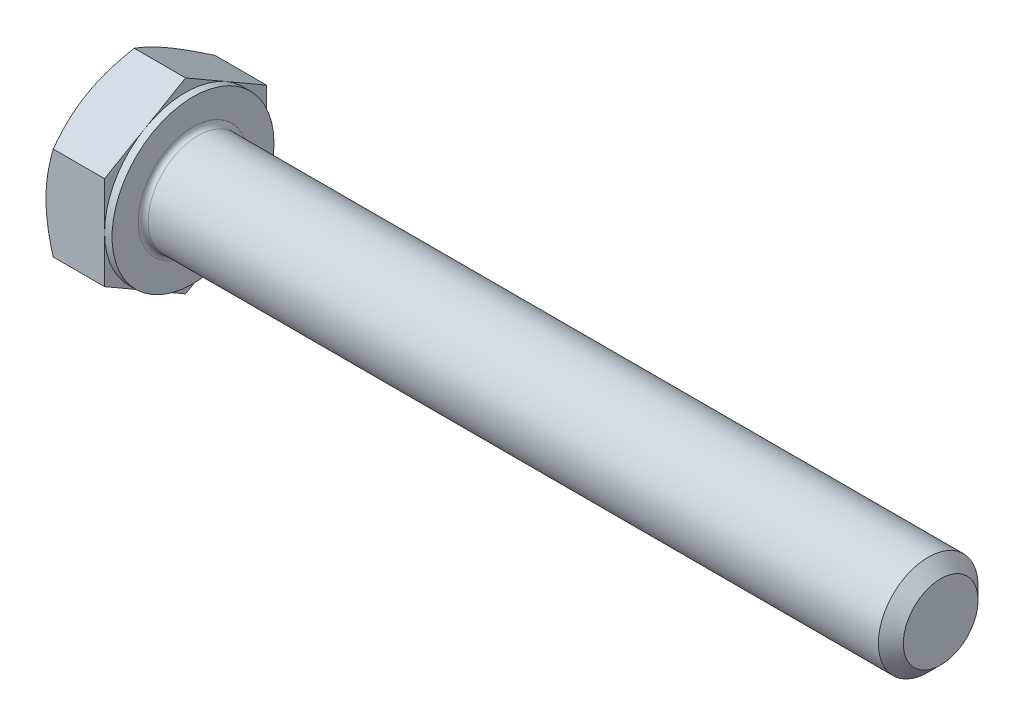
SolidWorks part; units mm, degrees
extrude "Base-Extrude" add sketch "Sketch1" along normal blind 5.3
sketch "Sketch1" plane through (0, 0, 0) normal (1, 0, 0) x (0, 0, -1)
  line L0 (6.5, 3.7528) -> (6.5, -3.7528)
  line L1 (-6.5, 3.7528) -> (-6.5, -3.7528)
  line L2 (6.5, -3.7528) -> (0, -7.5056)
  line L3 (0, -7.5056) -> (-6.5, -3.7528)
  line L4 (6.5, 3.7528) -> (0, 7.5056)
  line L5 (0, 7.5056) -> (-6.5, 3.7528)
revolve "Cut-Revolve1" cut sketch "Sketch3" angle 360 about L6
sketch "Sketch3" plane through (0, 0, 0) normal (0, 0, 1) x (1, 0, 0)
  line L0 (0, 6.5) -> (3.4673, 12.5056)
  line L1 (0, 7.5056) -> (0, 3.7528) construction
  line L2 (3.4673, 12.5056) -> (3.4673, 17.5056)
  line L3 (3.4673, 17.5056) -> (-10, 17.5056)
  line L4 (-10, 17.5056) -> (-10, 6.5)
  line L5 (-10, 6.5) -> (0, 6.5)
  line L6 (0, 0) -> (99.06, 0) construction
  line L7 (5.3, 7.5056) -> (0, 7.5056) construction
ref_plane "Front" through (0, 0, 0) normal (0, 0, 1) x (1, 0, 0)
ref_plane "Top" through (0, 0, 0) normal (0, 1, 0) x (1, 0, 0)
ref_plane "Right" through (0, 0, 0) normal (1, 0, 0) x (0, 0, -1)
sketch "Sketch2" plane through (0, 0, 0) normal (0, 0, 1) x (1, 0, 0)
  line L0 (0, 3.7528) -> (0, -3.7528) construction
  line L1 (0, 0) -> (65.3, 0)
  line L2 (0, 0) -> (0, 4)
  line L3 (0, 4) -> (7.7917, 4)
  line L4 (65.3, 0) -> (65.3, 2.9175)
  line L5 (5.3, 7.5056) -> (5.3, 3.7528) construction
  line L7 (0, 0) -> (96.52, 0) construction
  line L8 (65.3, -2.9175) -> (7.7917, -4) construction
  line L9 (0, -4) -> (7.7917, -4) construction
  line L10 (6.55, 15.24) -> (6.55, -1.27) construction
  line L11 (43.3, 15.24) -> (43.3, -1.27) construction
  line L12 (5.3, 3.7528) -> (5.3, -3.7528) construction
  line L13 (7.7917, 4) -> (65.3, 4)
  line L14 (65.3, 4) -> (65.3, 2.9175)
revolve "Boss-Revolve1" add sketch "Sketch2" angle 360 about L7
cosmetic thread "Helix1" parameters "Thread_length"=22, "Thread_minor"=5.835
sketch "Sketch5" plane through (0, 0, 0) normal (0, 0, 1) x (1, 0, 0)
  line L0 (5.3, 6.5) -> (1.8327, 12.5056)
  line L1 (5.3, 7.5056) -> (5.3, 3.7528) construction
  line L2 (1.8327, 12.5056) -> (1.8327, 17.5056)
  line L3 (1.8327, 17.5056) -> (11.8327, 17.5056)
  line L4 (11.8327, 17.5056) -> (11.8327, 6.5)
  line L5 (11.8327, 6.5) -> (5.3, 6.5)
  line L7 (5.3, 7.5056) -> (0.5806, 7.5056) construction
  line L8 (0, 0) -> (99.06, 0) construction
  line L9 (0, 0) -> (99.06, 0) construction
revolve "Cut-Revolve2" cut sketch "Sketch5" angle 360 about L8
sketch "Sketch4" plane through (0, 0, 0) normal (0, 0, 1) x (1, 0, 0)
  line L1 (5.3, 7.5056) -> (5.3, 3.7528) construction
  line L2 (5.3, 6.5) -> (4.7, 6.5)
  line L3 (5.3, 6.5) -> (5.3, 17.5056)
  line L4 (5.3, 17.5056) -> (4.7, 17.5056)
  line L5 (0, 0) -> (95.25, 0) construction
  line L6 (0, 0) -> (96.52, 0) construction
  line L7 (4.7, 6.5) -> (4.7, 17.5056)
  line L8 (4.7194, 7.5056) -> (0.5806, 7.5056) construction
revolve "Cut-Revolve3" cut sketch "Sketch4" angle 360 about L5
chamfer "Chamfer" distance 1 angle 45 1 edges at (65.3, 0, 4)
fillet "Fillet" radius 0.4 1 edges at (5.3, 0, -4)
sketch "Sketch6" plane through (0, 0, 0) normal (0, 0, 1) x (1, 0, 0)
  line L0 (43.3, -2.9175) -> (42.675, -4)
  line L1 (43.3, -2.9175) -> (43.925, -4)
  line L2 (43.925, -4) -> (43.925, -5)
  line L3 (-3.175, 0) -> (5.1513, 0) construction
  line L5 (43.925, -5) -> (42.675, -5)
  line L6 (42.675, -5) -> (42.675, -4)
revolve "Cut-Revolve4" [suppressed] cut sketch "Sketch6" angle 360 about L3
pattern_linear "LPattern1" [suppressed]
equation "\"D3@Sketch1\" = \"s@Sketch1\" / 2"
equation "\"D4@Sketch1\" = \"D3@Sketch1\""
equation "\"D5@Sketch1\" = \"D4@Sketch1\""
equation "\"Thread_minor@Helix1\" = \"Minor_dia@Sketch2\""
equation "\"D1@Sketch3\" = \"s@Sketch1\" / 2"
equation "\"D1@Sketch5\" = \"s@Sketch1\" / 2"
equation "\"Head_ch_ang@Sketch5\" = \"Head_ch_ang@Sketch3\""
equation "\"D1@Sketch4\" = \"s@Sketch1\""
equation "\"Thread_length@Helix1\" = ((sgn( (\"l@Sketch2\" - \"p@Sketch2\" ) - \"h@Sketch2\" )-1)*( (\"l@Sketch2\" - \"p@Sketch2\" ) - \"h@Sketch2\" ))/-2+ \"h@Sketch2\""
equation "\"Thread_minor@Sketch6\" = \"Minor_dia@Sketch2\""
equation "\"Diameter@Sketch6\" = \"m@Sketch2\""
equation "\"Overcut@Sketch6\" = \"m@Sketch2\" * 1.25"
equation "\"Start@Sketch6\" = \"k@Base-Extrude\" + \"l@Sketch2\" - \"Thread_length@Helix1\"  '---Non-countersunk---"
equation "\"Num_threads@LPattern1\" = int( \"Thread_length@Helix1\" / \"p@Sketch2\" + 0.999 )  + 1"
equation "\"Advance@LPattern1\" = \"Thread_length@Helix1\" /  (\"Num_threads@LPattern1\" - 1) 'relax it"
equation "\"Num_threads@LPattern1\" = \"Num_threads@LPattern1\" - sgn( \"Num_threads@LPattern1\" - 1) '---chamfered tips oxxx---"
equation "\"Minor_dia@Sketch2\" = \"m@Sketch2\"-\"p@Sketch2\" * 1.732"
equation "\"D1@Chamfer\" = \"p@Sketch2\"*0.8"
